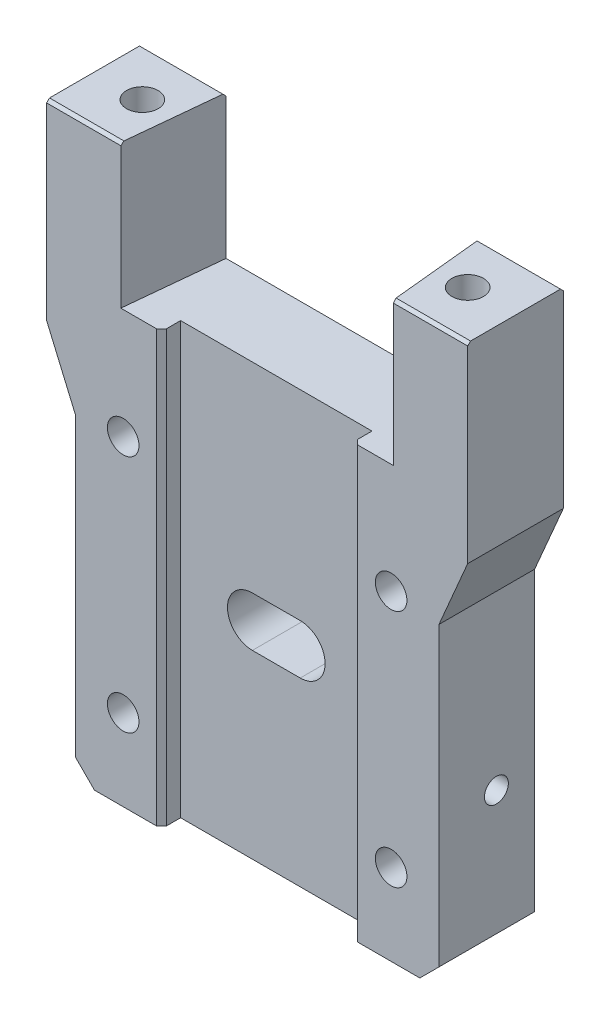
from build123d import *

# Parameters (mm, degrees)
SKETCH1_W             = 44
SKETCH1_H             = 60
BOSS_EXTRUDE1_DEPTH   = 10
CUT_EXTRUDE4_DEPTH    = 15
SKETCH2_W             = 20
SKETCH2_H             = 60
CUT_EXTRUDE1_DEPTH    = 2
M4_TAPPED_HOLE1_D     = 3.3
M4_TAPPED_HOLE1_DEPTH = 10.1
M4_TAPPED_HOLE1_TIP   = 0.991420021
M4_TAPPED_HOLE2_D     = 3.3
M4_TAPPED_HOLE2_DEPTH = 10.1
M4_TAPPED_HOLE2_TIP   = 0.991420021
M3_TAPPED_HOLE2_D     = 2.5
M3_TAPPED_HOLE2_DEPTH = 7.5
M3_TAPPED_HOLE2_TIP   = 0.751075774
CHAMFER3_SIZE         = 0.3
CHAMFER4_SIZE         = 0.5
CUT_EXTRUDE5_DEPTH    = 39.522720569
CHAMFER5_SIZE         = 2
CUT_EXTRUDE6_DEPTH    = 39.522720569


with BuildPart() as part:
    # Sketch1 → Boss-Extrude1 (new body)
    with BuildSketch(Plane.XY):
        Rectangle(SKETCH1_W, SKETCH1_H)
    extrude(amount=BOSS_EXTRUDE1_DEPTH)

    # Sketch13 → Cut-Extrude4 (cut)
    with BuildSketch(Plane(origin=(0, 30, 0), x_dir=(1, 0, 0), z_dir=(0, 1, 0))):
        Polygon((13.25, 0), (14.25, -10), (-14.25, -10), (-13.25, 0), align=None)
    extrude(amount=-CUT_EXTRUDE4_DEPTH, mode=Mode.SUBTRACT)

    # Sketch2 → Cut-Extrude1 (cut)
    with BuildSketch(Plane.XY.offset(10)):
        Rectangle(SKETCH2_W, SKETCH2_H)
    extrude(amount=-CUT_EXTRUDE1_DEPTH, mode=Mode.SUBTRACT)

    # M4 Tapped Hole1
    with Locations(Plane(origin=(0, 30, 0), x_dir=(1, 0, 0), z_dir=(0, 1, 0))):
        with Locations((-17, -5), (17, -5)):
            Hole(M4_TAPPED_HOLE1_D / 2, depth=M4_TAPPED_HOLE1_DEPTH)
            with Locations((0, 0, -(M4_TAPPED_HOLE1_DEPTH + M4_TAPPED_HOLE1_TIP / 2))):  # 118° drill point
                Cone(0, M4_TAPPED_HOLE1_D / 2, M4_TAPPED_HOLE1_TIP, mode=Mode.SUBTRACT)

    # M4 Tapped Hole2
    with Locations(Plane.XY.offset(10)):
        with Locations((-14, -21.5), (14, -21.5), (-14, 3.5), (14, 3.5)):
            Hole(M4_TAPPED_HOLE2_D / 2, depth=M4_TAPPED_HOLE2_DEPTH)
            with Locations((0, 0, -(M4_TAPPED_HOLE2_DEPTH + M4_TAPPED_HOLE2_TIP / 2))):  # 118° drill point
                Cone(0, M4_TAPPED_HOLE2_D / 2, M4_TAPPED_HOLE2_TIP, mode=Mode.SUBTRACT)

    # M3 Tapped Hole2
    with Locations(Plane(origin=(22, 0, 0), x_dir=(0, 0, -1), z_dir=(1, 0, 0))):
        with Locations((-4, -15)):
            Hole(M3_TAPPED_HOLE2_D / 2, depth=M3_TAPPED_HOLE2_DEPTH)
            with Locations((0, 0, -(M3_TAPPED_HOLE2_DEPTH + M3_TAPPED_HOLE2_TIP / 2))):  # 118° drill point
                Cone(0, M3_TAPPED_HOLE2_D / 2, M3_TAPPED_HOLE2_TIP, mode=Mode.SUBTRACT)

    # Chamfer3
    chamfer3_edges = [part.edges().sort_by_distance(p)[0] for p in [
        (-17.625, 30, 0),
        (-18.125, 30, 10),
        (17.625, 30, 0),
        (18.125, 30, 10),
    ]]
    chamfer(chamfer3_edges, length=CHAMFER3_SIZE)

    # Chamfer4
    chamfer4_edges = [part.edges().sort_by_distance(p)[0] for p in [
        (10, -7.5, 10),
        (-10, -7.5, 10),
    ]]
    chamfer(chamfer4_edges, length=CHAMFER4_SIZE)

    # Sketch14 → Cut-Extrude5 (cut, through all)
    with BuildSketch(Plane.XY.offset(10)):
        Polygon((-19, -30), (-19, 3), (-22, 10), (-22, -30), align=None)
        Polygon((19, -30), (19, 3), (22, 10), (22, -30), align=None)
    extrude(amount=-CUT_EXTRUDE5_DEPTH, mode=Mode.SUBTRACT)

    # Chamfer5
    chamfer5_edges = [part.edges().sort_by_distance(p)[0] for p in [
        (-19, -30, 5),
        (19, -30, 5),
    ]]
    chamfer(chamfer5_edges, length=CHAMFER5_SIZE)

    # Sketch15 → Cut-Extrude6 (cut, through all)
    with BuildSketch(Plane(origin=(0, 0, 0), x_dir=(-1, 0, 0), z_dir=(0, 0, -1))):
        with BuildLine():
            Line((-2.5, -5.9), (2.5, -5.9))
            ThreePointArc((2.5, -5.9), (5.1, -8.5), (2.5, -11.1))
            Line((2.5, -11.1), (-2.5, -11.1))
            ThreePointArc((-2.5, -11.1), (-5.1, -8.5), (-2.5, -5.9))
        make_face()
    extrude(amount=-CUT_EXTRUDE6_DEPTH, mode=Mode.SUBTRACT)


solid = part.part
